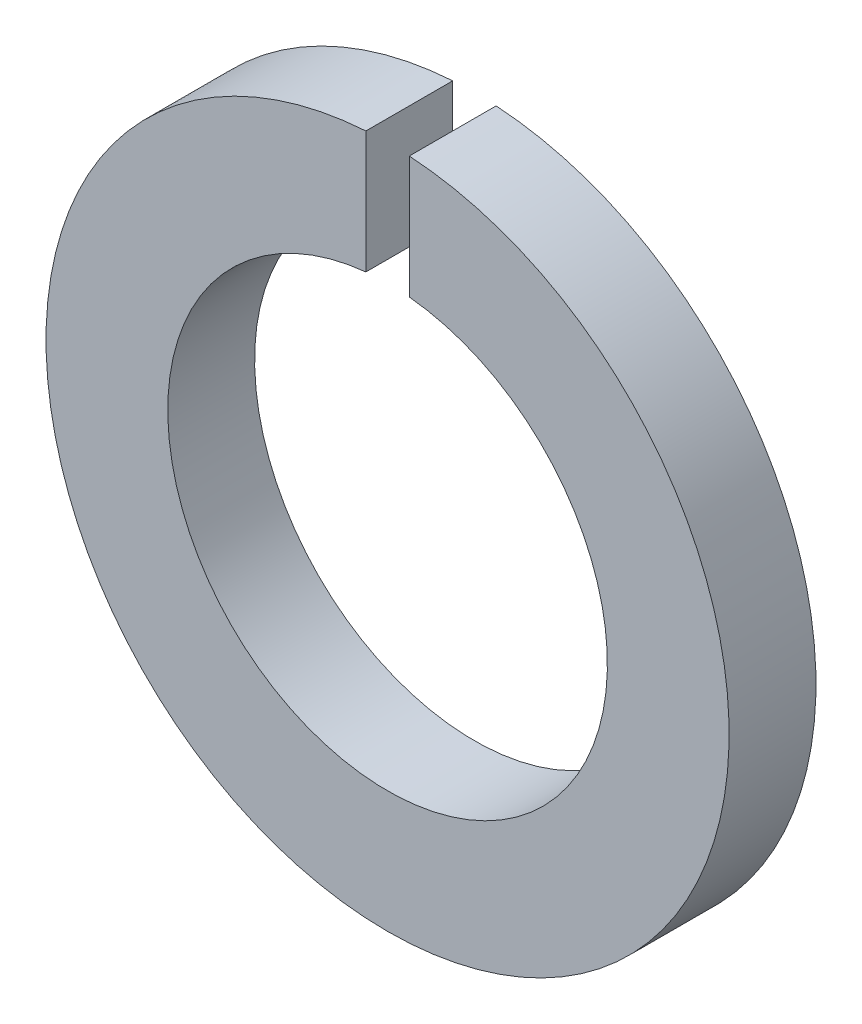
SolidWorks part; units mm, degrees
ref_plane "前视基准面" through (0, 0, 0) normal (0, 0, 1) x (1, 0, 0)
ref_plane "上视基准面" through (0, 0, 0) normal (0, 1, 0) x (1, 0, 0)
ref_plane "右视基准面" through (0, 0, 0) normal (1, 0, 0) x (0, 0, -1)
sketch "尺寸草图" plane through (0, 0, 0) normal (0, 0, 1) x (1, 0, 0)
  line L0 (0, 0) -> (0, 14.803) construction
  line L1 (-0.8, 12.5604) -> (-0.8, 8.0604)
  line L2 (0.8, 12.5604) -> (0.8, 8.0604)
  line L3 (0, 0) -> (3.2, 0) construction
  arc A0 (-0.8, 12.5604) -> (0.8, 12.5604) centre (0, 0) ccw
  arc A2 (-0.8, 8.0604) -> (0.8, 8.0604) centre (0, 0) ccw
  dimension "d" = 16.2
  dimension "m" = 1.6
  dimension "D4" = 0.8
  dimension "b" = 4.5
  dimension "s" = 3.2
extrude "拉伸1" add sketch "尺寸草图" along normal blind 3.2
